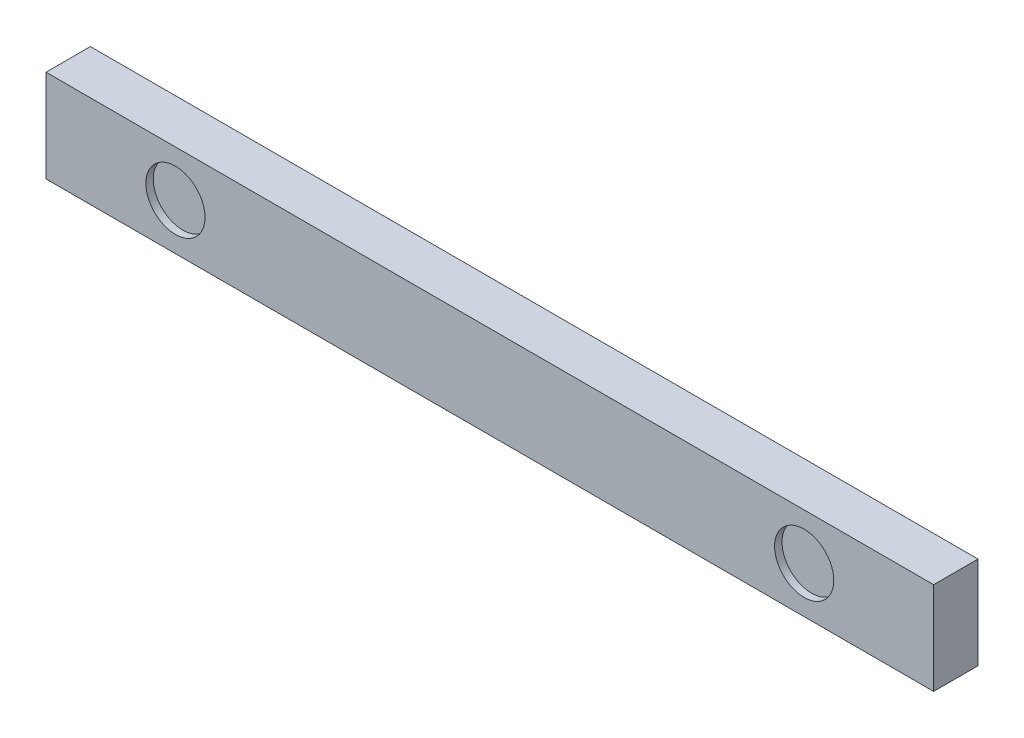
from build123d import *

# Parameters (mm, degrees)
SKETCH_1_W          = 240
SKETCH_1_H          = 25
EXTRUDE_1_DEPTH     = 12
SKETCH_2_R          = 8
CUT_EXTRUDE_1_DEPTH = 2


with BuildPart() as part:
    # 草图1 → 凸台-拉伸1 (new body)
    with BuildSketch(Plane.XY):
        Rectangle(SKETCH_1_W, SKETCH_1_H)
    extrude(amount=EXTRUDE_1_DEPTH)

    # 草图2 → 切除-拉伸1 (cut)
    with BuildSketch(Plane.XY.offset(12)):
        with Locations((85, 0)):
            Circle(SKETCH_2_R)
        with Locations((-85, 0)):
            Circle(SKETCH_2_R)
    extrude(amount=-CUT_EXTRUDE_1_DEPTH, mode=Mode.SUBTRACT)


solid = part.part
